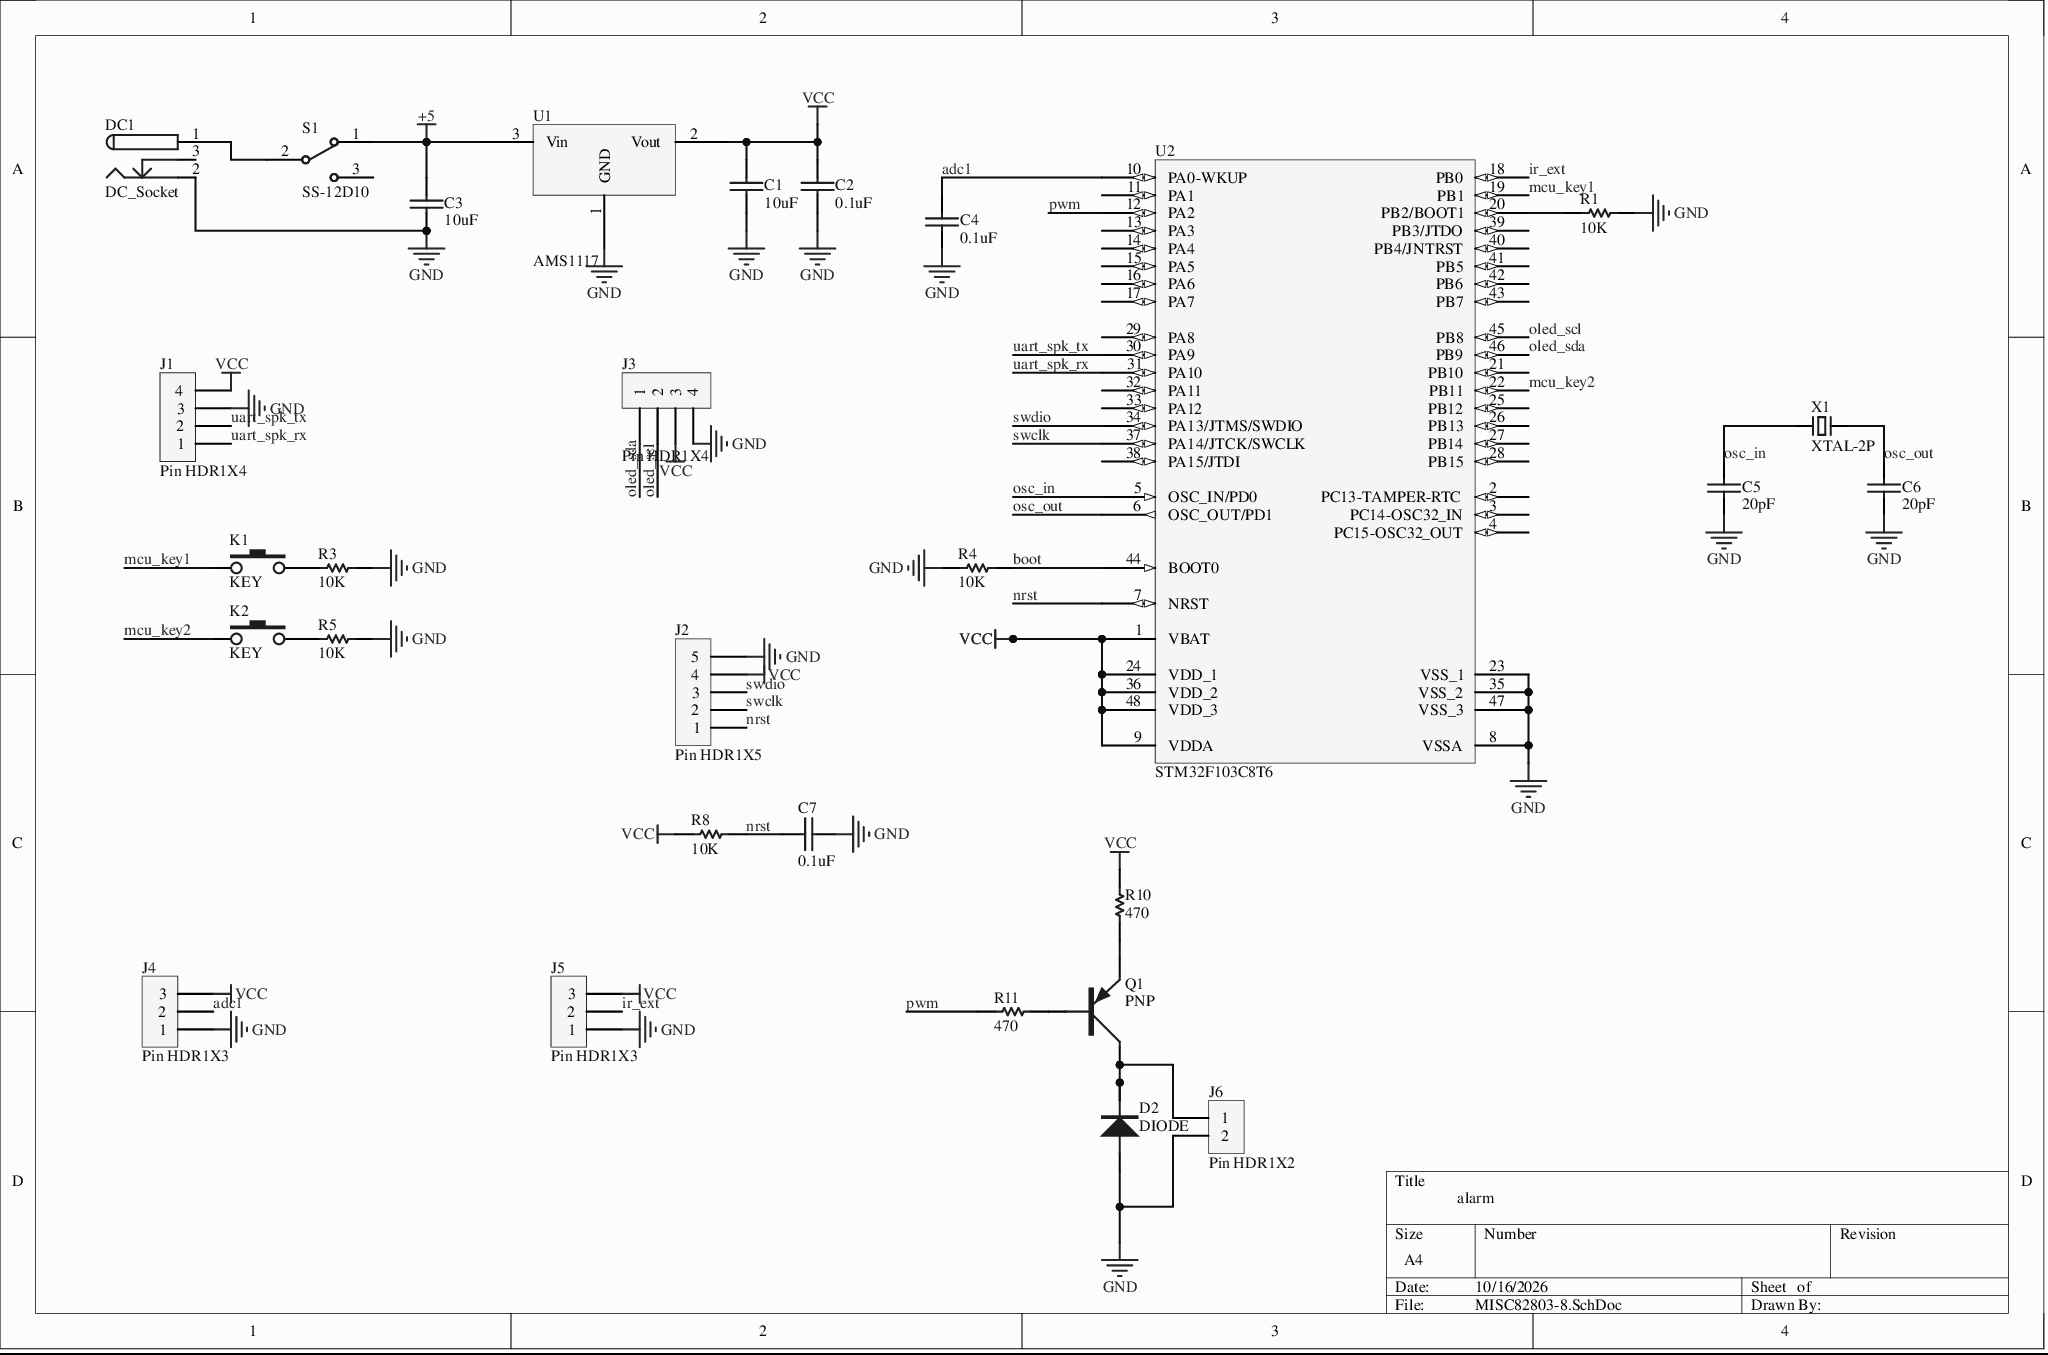
[diagram p0: MISC82803-8.SchDoc]
# Altium project MISC82803-4.PrjPCB
1 sheet, 29 parts. Net scope: global (net labels, ports and power ports of the same name join across sheets).
Board file: MISC82803.PcbDoc

## Sheet MISC82803-8.SchDoc
size A4

### Parts
C1  10uF  [0603C]
C2  0.1uF  [0603C]
C3  10uF  [0603C]
C4  0.1uF  [0603C]
C5  20pF  [0603C]
C6  20pF  [0603C]
C7  0.1uF  [0603C]
D2  DIODE  [SOD-123]
DC1  DC_Socket  [DC-002]
J1  Pin HDR1X4  [Pin HDR1X4/2.54mm-S]
J2  Pin HDR1X5  [Pin HDR1X5/2.54mm-S]
J3  Pin HDR1X4  [Pin HDR1X4/2.54mm-S]
J4  Pin HDR1X3  [Pin HDR1X3/2.54mm-S]
J5  Pin HDR1X3  [Pin HDR1X3/2.54mm-S]
J6  Pin HDR1X2  [Pin HDR1X2/2.54mm-S]
K1  KEY  [DIP-3X6X4.3]
K2  KEY  [DIP-3X6X4.3]
Q1  PNP  [SOT-23]
R1  10K  [0603R]
R3  10K  [0603R]
R4  10K  [0603R]
R5  10K  [0603R]
R8  10K  [0603R]
R10  470  [0603R]
R11  470  [0603R]
S1  SS-12D10  [SS-12D10]
U1  AMS1117  [SOT223]
U2  STM32F103C8T6  [LQFP48 7X7]
X1  XTAL-2P  [OSC HC-49S]

### Nets
+5: C3.2 S1.1 U1.3(Vin)
GND: C1.1 C2.1 C3.1 C4.1 C5.1 C6.1 C7.1 D2.A DC1.2 J1.3 J2.5 J3.4 J4.1 J5.1 J6.2 R1.1 R3.1 R4.2 R5.1 U1.1(GND) U2.8(VSSA) U2.23(VSS_1) U2.35(VSS_2) U2.47(VSS_3)
VCC: C1.2 C2.2 J1.4 J2.4 J3.3 J4.3 J5.3 R8.2 R10.1 U1.2(Vout) U2.1(VBAT) U2.9(VDDA) U2.24(VDD_1) U2.36(VDD_2) U2.48(VDD_3)
adc1: C4.2 J4.2 U2.10(PA0-WKUP)
boot: R4.1 U2.44(BOOT0)
ir_ext: J5.2 U2.18(PB0)
mcu_key1: K1.1 U2.19(PB1)
mcu_key2: K2.1 U2.22(PB11)
nrst: C7.2 J2.1 R8.1 U2.7(NRST)
oled_scl: J3.2 U2.45(PB8)
oled_sda: J3.1 U2.46(PB9)
osc_in: C5.2 U2.5(OSC_IN/PD0) X1.1
osc_out: C6.2 U2.6(OSC_OUT/PD1) X1.2
pwm: R11.1 U2.12(PA2)
swclk: J2.2 U2.37(PA14/JTCK/SWCLK)
swdio: J2.3 U2.34(PA13/JTMS/SWDIO)
uart_spk_rx: J1.1 U2.31(PA10)
uart_spk_tx: J1.2 U2.30(PA9)
NetD2_K: D2.K J6.1 Q1.C
NetDC1_1: DC1.1 S1.2
NetK1_3: K1.3 R3.2
NetK2_3: K2.3 R5.2
NetQ1_B: Q1.B R11.2
NetQ1_E: Q1.E R10.2
NetR1_2: R1.2 U2.20(PB2/BOOT1)

Not connected (* = marked no-connect by the designer): DC1 3; S1 3; U2 2(PC13-TAMPER-RTC) 3(PC14-OSC32_IN) 4(PC15-OSC32_OUT) 11(PA1) 13(PA3) 14(PA4) 15(PA5) 16(PA6) 17(PA7) 21(PB10) 25(PB12) 26(PB13) 27(PB14) 28(PB15) 29(PA8) 32(PA11) 33(PA12) 38(PA15/JTDI) 39(PB3/JTDO) 40(PB4/JNTRST) 41(PB5) 42(PB6) 43(PB7)

### Notes on the sheet
- alarm

### Library data of the parts
C1-C7 = CAP: Non-polar capacitor
D2 = DIODE: General diode
Q1 = PNP: PNP transistor
R1 R3-R5 R8 R10 R11 = RES
U1 = AMS1117: Three-terminal voltage regulator
X1 = XTAL-2P: 2-pin passive crystal oscillator